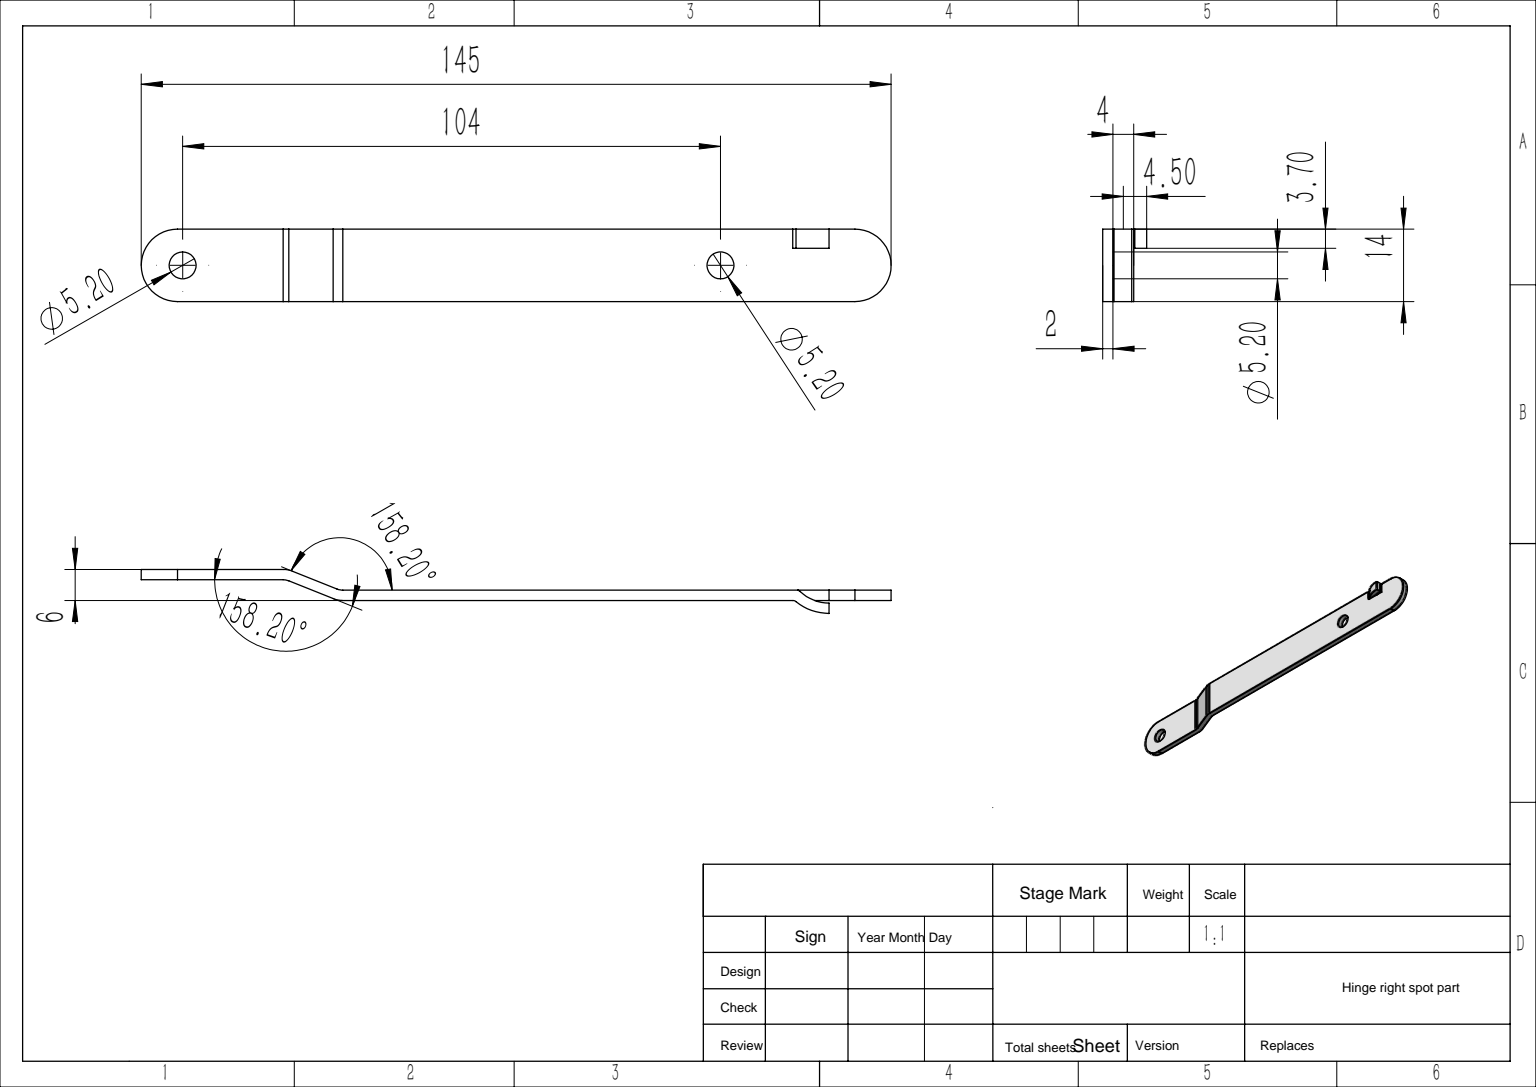
SolidWorks part; units mm, degrees
material "普通碳钢"
ref_plane "Front Plane" through (0, 0, 0) normal (0, 0, 1) x (1, 0, 0)
ref_plane "Top Plane" through (0, 0, 0) normal (0, 1, 0) x (1, 0, 0)
ref_plane "Right Plane" through (0, 0, 0) normal (1, 0, 0) x (0, 0, -1)
sketch "Sketch1" plane through (0, 0, 0) normal (0, 0, 1) x (1, 0, 0)
  line L0 (0, 0) -> (27.4223, 0)
  line L1 (28.5364, 0.2146) -> (37.106, 3.6424)
  line L2 (38.9629, 4) -> (145, 4)
  line L3 (0, -2) -> (27.4223, -2)
  line L4 (29.2792, -1.6424) -> (37.8487, 1.7854)
  line L5 (38.9629, 2) -> (145, 2)
  line L6 (0, 0) -> (0, -2)
  line L7 (145, 4) -> (145, 2)
  arc A0 (38.9629, 4) -> (37.106, 3.6424) centre (38.9629, -1) ccw
  arc A1 (28.5364, 0.2146) -> (27.4223, 0) centre (27.4223, 3) cw
  arc A2 (29.2792, -1.6424) -> (27.4223, -2) centre (27.4223, 3) cw
  arc A3 (38.9629, 2) -> (37.8487, 1.7854) centre (38.9629, -1) ccw
  point P7 (38, 4)
  point P10 (28, 0)
  dimension "D5" = 5
  dimension "D6" = 3
  dimension "D1" = 145
  dimension "D2" = 28
  dimension "D3" = 4
  dimension "D4" = 10
  dimension "D7" = 2
extrude "Extrude1" add sketch "Sketch1" along normal mid plane 14
sketch "Sketch2" plane through (0, 0, 0) normal (0, 1, 0) x (1, 0, 0)
  line L0 (0, -7) -> (0, 7) construction
  line L1 (145, -7) -> (145, 7) construction
  line L2 (138, 7) -> (138, 13.5023)
  line L3 (138, 13.5023) -> (156.332, 13.5023)
  line L4 (156.332, 13.5023) -> (156.332, -14.2627)
  line L5 (156.332, -14.2627) -> (138, -14.2627)
  line L6 (138, -14.2627) -> (138, -7)
  line L7 (7, 7) -> (7, 12.6636)
  line L8 (7, 12.6636) -> (-7.0971, 12.6636)
  line L9 (-7.0971, 12.6636) -> (-7.0971, -11.0535)
  line L10 (-7.0971, -11.0535) -> (7, -11.0535)
  line L11 (7, -11.0535) -> (7, -7)
  arc A0 (7, 7) -> (7, -7) centre (7, 0) ccw
  arc A1 (138, -7) -> (138, 7) centre (138, 0) ccw
  circle A2 centre (8, 0) radius 2.6
  circle A3 centre (112, 0) radius 2.6
  dimension "D1" = 5.2
  dimension "D3" = 5.2
  dimension "D2" = 8
  dimension "D4" = 104
extrude "Extrude2" cut sketch "Sketch2" against normal through all and the other way through all
sketch "Sketch5" plane through (0, 4, 0) normal (0, 1, 0) x (1, 0, 0)
  line L5 (138, 7) -> (38.9629, 7) construction
  line L6 (127, 7) -> (133, 7)
  line L7 (127, 7) -> (127, 3.3)
  line L8 (127, 3.3) -> (133, 3.3)
  line L9 (133, 7) -> (133, 3.3)
  circle A0 centre (112, 0) radius 2.6 construction
  dimension "D4" = 6
  dimension "D5" = 3.7
  dimension "D6" = 15
extrude "Extrude5" cut sketch "Sketch5" against normal through all
sketch "Sketch6" plane through (0, 0, -7) normal (0, 0, 1) x (1, 0, 0)
  line L1 (138, 4) -> (38.9629, 4) construction
  line L2 (133, 4) -> (133, 2) construction
  line L3 (125.9784, 4) -> (124.3136, 4)
  line L5 (127, 2) -> (127, 4) construction
  line L6 (138, 2) -> (145, 2) construction
  line L7 (38.9629, 2) -> (138, 2) construction
  line L8 (124.3136, 2) -> (126.7308, 2)
  line L10 (133, 4.5) -> (133, 6.5)
  line L11 (124.3136, 4) -> (124.3136, 2)
  arc A0 (126.6104, 4.225) -> (133, 6.5) centre (133, -3.6106) cw
  arc A1 (127.4189, 2.2744) -> (133, 4.5) centre (133, -3.6106) cw
  arc A2 (126.5115, 1.2557) -> (133, 4.5) centre (133, -3.6106) cw construction
  arc A3 (125.9784, 4) -> (126.6104, 4.225) centre (125.9784, 5) ccw
  arc A4 (124.9115, 2.4557) -> (133, 6.5) centre (133, -3.6106) cw construction
  arc A5 (126.7308, 2) -> (127.4189, 2.2744) centre (126.7308, 3) ccw
  dimension "D3" = 1
  dimension "D4" = 2.6864
  dimension "D1" = 4.5
  dimension "D2" = 2
extrude "Extrude6" add sketch "Sketch6" along normal blind 3.7
